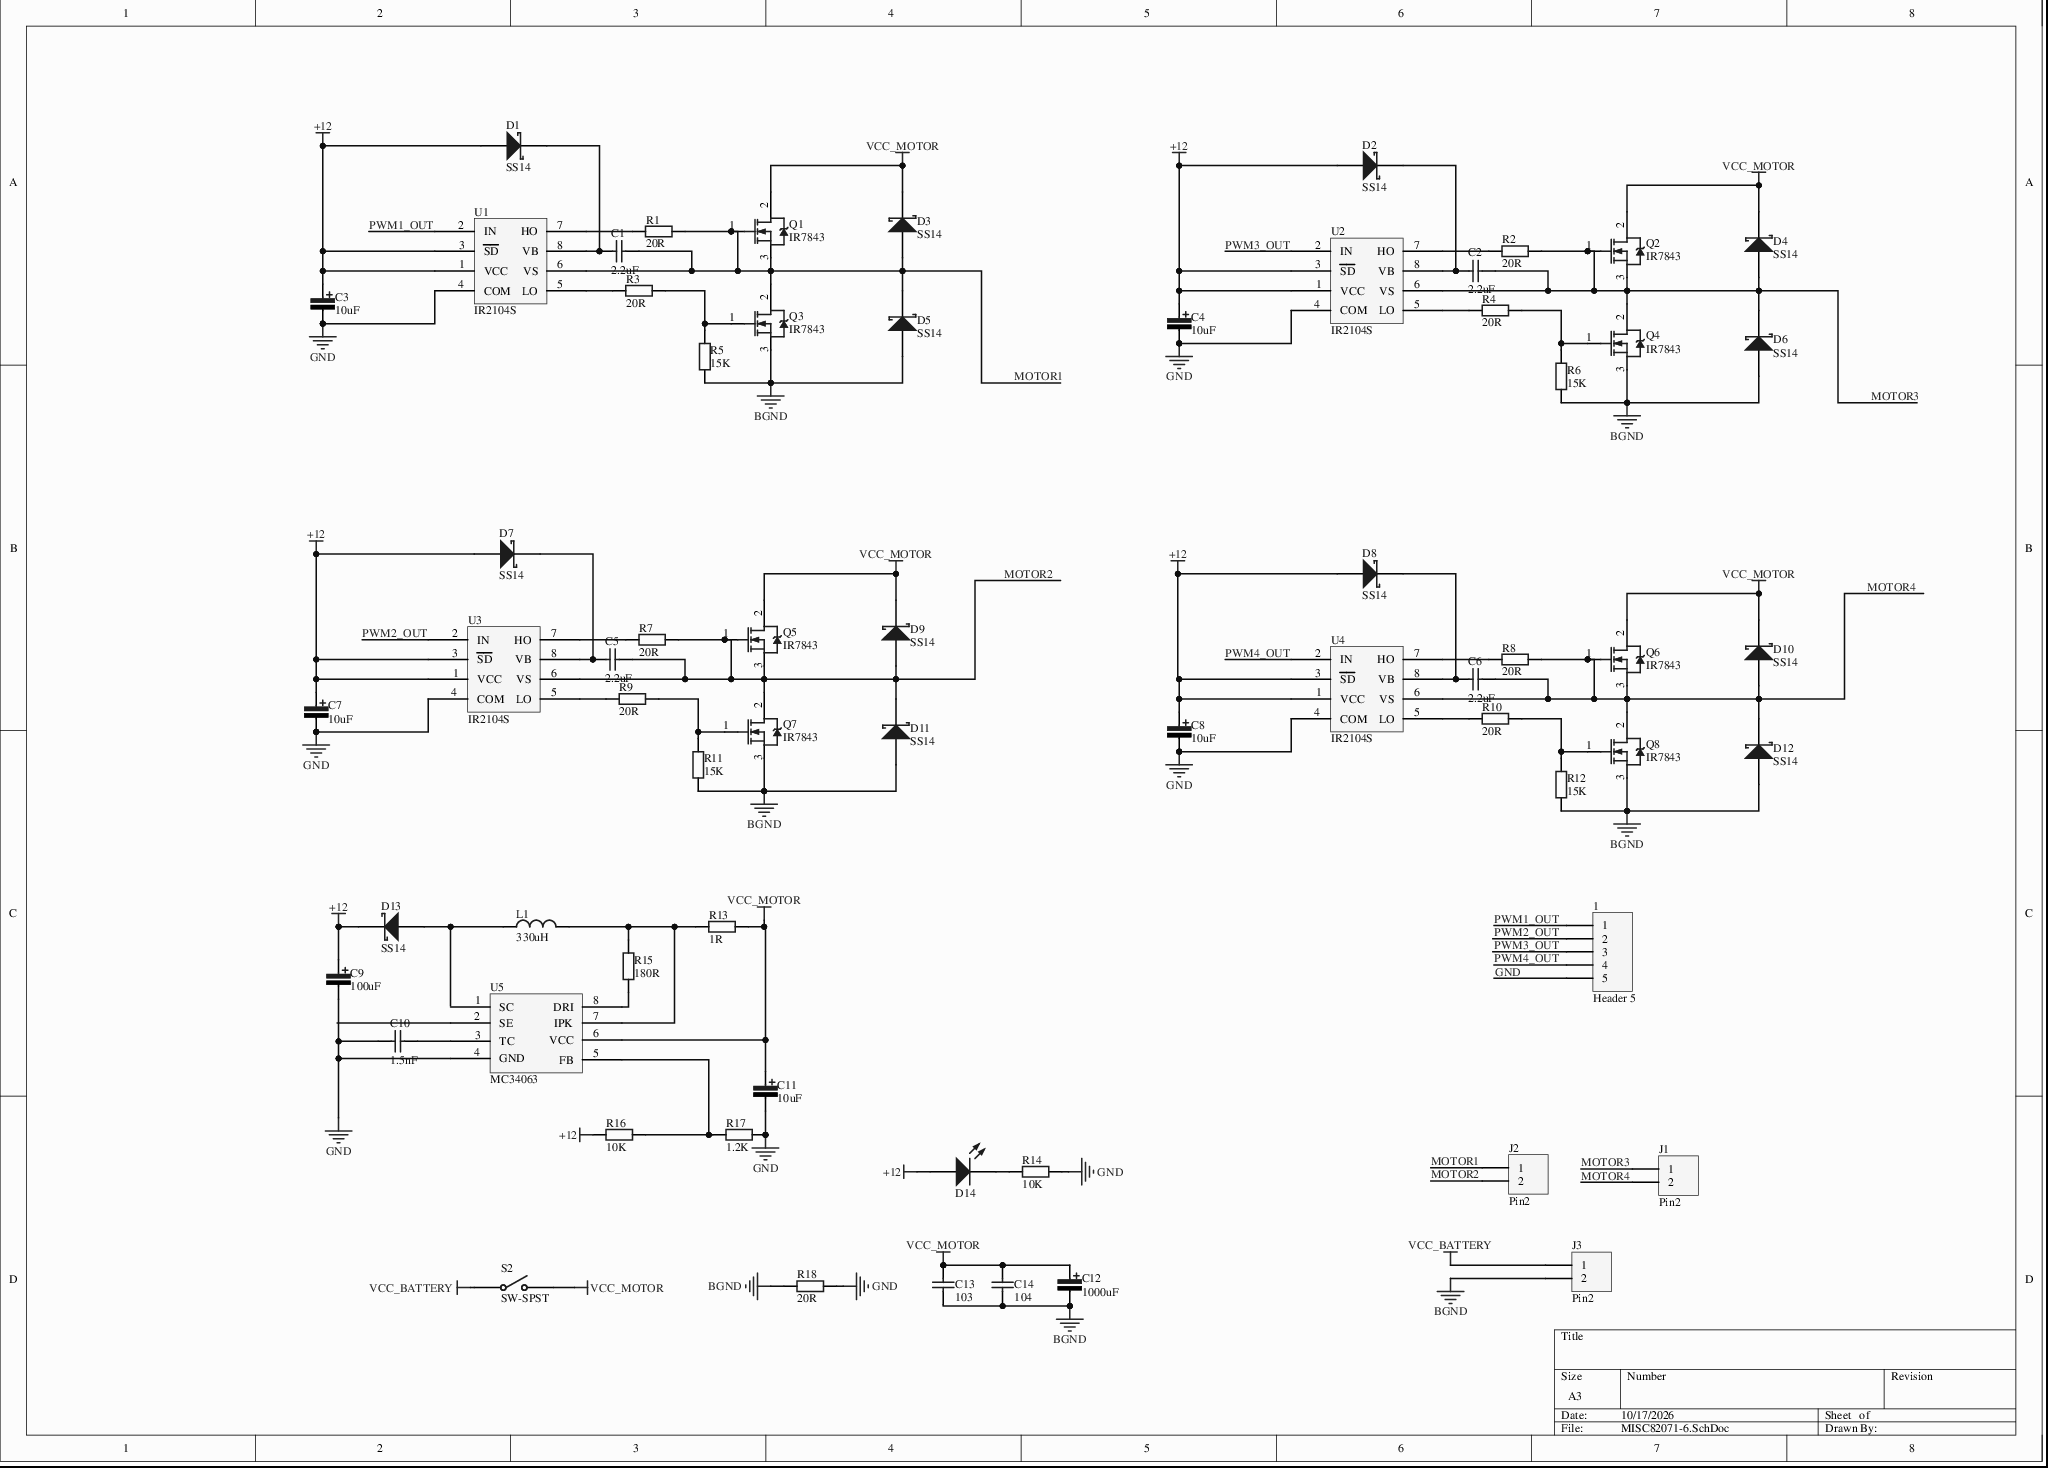
[diagram p0: MISC82071-6.SchDoc]
# Altium project MISC82071-6.PrjPcb
1 sheet, 65 parts. Net scope: global (net labels, ports and power ports of the same name join across sheets).
Board file: MISC82071.PcbDoc

## Sheet MISC82071-6.SchDoc
size A3; SheetNumber: 1; SheetTotal: 1

### Parts
1  Header 5  [HDR1X5]
C1  value 2.2uF  [my0603]  (hidden comment: Cap)
C2  value 2.2uF  [my0603]  (hidden comment: Cap)
C3  value 10uF  [CAP-3528]  (hidden comment: Cap Pol)
C4  value 10uF  [CAP-3528]  (hidden comment: Cap Pol)
C5  value 2.2uF  [my0603]  (hidden comment: Cap)
C6  value 2.2uF  [my0603]  (hidden comment: Cap)
C7  value 10uF  [CAP-3528]  (hidden comment: Cap Pol)
C8  value 10uF  [CAP-3528]  (hidden comment: Cap Pol)
C9  value 100uF  [CAP-3528]  (hidden comment: Cap Pol)
C10  value 1.5nF  [my0603]  (hidden comment: Cap)
C11  value 10uF  [CAP-3528]  (hidden comment: Cap Pol)
C12  value 1000uF  [CM A(3*5.4)]  (hidden comment: Cap Pol)
C13  value 103  [my0603]  (hidden comment: Cap)
C14  value 104  [my0603]  (hidden comment: Cap)
D1  Type: SS14  [DIODE-SMA]  (hidden comment: D-Schottky)
D2  Type: SS14  [DIODE-SMA]  (hidden comment: D-Schottky)
D3  Type: SS14  [DIODE-SMA]  (hidden comment: D-Schottky)
D4  Type: SS14  [DIODE-SMA]  (hidden comment: D-Schottky)
D5  Type: SS14  [DIODE-SMA]  (hidden comment: D-Schottky)
D6  Type: SS14  [DIODE-SMA]  (hidden comment: D-Schottky)
D7  Type: SS14  [DIODE-SMA]  (hidden comment: D-Schottky)
D8  Type: SS14  [DIODE-SMA]  (hidden comment: D-Schottky)
D9  Type: SS14  [DIODE-SMA]  (hidden comment: D-Schottky)
D10  Type: SS14  [DIODE-SMA]  (hidden comment: D-Schottky)
D11  Type: SS14  [DIODE-SMA]  (hidden comment: D-Schottky)
D12  Type: SS14  [DIODE-SMA]  (hidden comment: D-Schottky)
D13  Type: SS14  [DIODE-SMA]  (hidden comment: D-Schottky)
D14  LED0  [0805]  (value not drawn)
J1  Pin2  [PCBComponent_1 - duplicate]
J2  Pin2  [PCBComponent_1 - duplicate]
J3  Pin2  [PCBComponent_1 - duplicate]
L1  value 330uH  [L-SMD-7]  (hidden comment: Inductor)
Q1  IR7843  [LR7843]
Q2  IR7843  [LR7843]
Q3  IR7843  [LR7843]
Q4  IR7843  [LR7843]
Q5  IR7843  [LR7843]
Q6  IR7843  [LR7843]
Q7  IR7843  [LR7843]
Q8  IR7843  [LR7843]
R1  value 20R  [0805]  (hidden comment: Res1)
R2  value 20R  [0805]  (hidden comment: Res1)
R3  value 20R  [0805]  (hidden comment: Res1)
R4  value 20R  [0805]  (hidden comment: Res1)
R5  value 15K  [0805]  (hidden comment: Res1)
R6  value 15K  [0805]  (hidden comment: Res1)
R7  value 20R  [0805]  (hidden comment: Res1)
R8  value 20R  [0805]  (hidden comment: Res1)
R9  value 20R  [0805]  (hidden comment: Res1)
R10  value 20R  [0805]  (hidden comment: Res1)
R11  value 15K  [0805]  (hidden comment: Res1)
R12  value 15K  [0805]  (hidden comment: Res1)
R13  value 1R  [0805]  (hidden comment: Res1)
R14  value 10K  [0805]  (hidden comment: Res1)
R15  value 180R  [0805]  (hidden comment: Res1)
R16  value 10K  [0805]  (hidden comment: Res1)
R17  value 1.2K  [0805]  (hidden comment: Res1)
R18  value 20R  [0805]  (hidden comment: Res1)
S2  SW-SPST  [SWITCH]
U1  IR2104S  [IR2104]
U2  IR2104S  [IR2104]
U3  IR2104S  [IR2104]
U4  IR2104S  [IR2104]
U5  MC34063  [MC34063]

### Nets
+12: C3.1 C4.1 C7.1 C8.1 C9.1 D1.1(A) D2.1(A) D7.1(A) D8.1(A) D13.2(K) D14.1(A) R16.1 U1.1(VCC) U1.3(~{SD}) U2.1(VCC) U2.3(~{SD}) U3.1(VCC) U3.3(~{SD}) U4.1(VCC) U4.3(~{SD})
BGND: C12.2 C13.1 C14.1 D5.1(A) D6.1(A) D11.1(A) D12.1(A) J3.2 Q3.3(S) Q4.3(S) Q7.3(S) Q8.3(S) R5.1 R6.1 R11.1 R12.1 R18.1
GND: 1.5 C3.2 C4.2 C7.2 C8.2 C9.2 C10.1 C11.2 R14.2 R17.2 R18.2 U1.4(COM) U2.4(COM) U3.4(COM) U4.4(COM) U5.4(GND)
VCC_BATTERY: J3.1 S2.1(COMMON)
VCC_MOTOR: C11.1 C12.1 C13.2 C14.2 D3.2(K) D4.2(K) D9.2(K) D10.2(K) Q1.2(D) Q2.2(D) Q5.2(D) Q6.2(D) R13.2 S2.2(NO) U5.6(VCC)
MOTOR1: C1.2 D3.1(A) D5.2(K) J2.1 Q1.1(G) Q1.3(S) Q3.2(D) R1.2 U1.6(VS)
MOTOR2: C5.2 D9.1(A) D11.2(K) J2.2 Q5.1(G) Q5.3(S) Q7.2(D) R7.2 U3.6(VS)
MOTOR3: C2.2 D4.1(A) D6.2(K) J1.1 Q2.1(G) Q2.3(S) Q4.2(D) R2.2 U2.6(VS)
MOTOR4: C6.2 D10.1(A) D12.2(K) J1.2 Q6.1(G) Q6.3(S) Q8.2(D) R8.2 U4.6(VS)
PWM1_OUT: 1.1 U1.2(IN)
PWM2_OUT: 1.2 U3.2(IN)
PWM3_OUT: 1.3 U2.2(IN)
PWM4_OUT: 1.4 U4.2(IN)
NetC1_1: C1.1 D1.2(K) U1.8(VB)
NetC2_1: C2.1 D2.2(K) U2.8(VB)
NetC5_1: C5.1 D7.2(K) U3.8(VB)
NetC6_1: C6.1 D8.2(K) U4.8(VB)
NetC10_2: C10.2 U5.3(TC)
NetD13_1: D13.1(A) L1.1
NetD14_2: D14.2(K) R14.1
NetL1_2: L1.2 R13.1 R15.2 U5.7(IPK)
NetQ3_1: Q3.1(G) R3.2 R5.2
NetQ4_1: Q4.1(G) R4.2 R6.2
NetQ7_1: Q7.1(G) R9.2 R11.2
NetQ8_1: Q8.1(G) R10.2 R12.2
NetR1_1: R1.1 U1.7(HO)
NetR2_1: R2.1 U2.7(HO)
NetR3_1: R3.1 U1.5(LO)
NetR4_1: R4.1 U2.5(LO)
NetR7_1: R7.1 U3.7(HO)
NetR8_1: R8.1 U4.7(HO)
NetR9_1: R9.1 U3.5(LO)
NetR10_1: R10.1 U4.5(LO)
NetR15_1: R15.1 U5.8(DRI)
NetR16_2: R16.2 R17.1 U5.5(FB)

Not connected (* = marked no-connect by the designer): U5 1(SC) 2(SE)

### Library data of the parts
1 = Header 5: Header, 5-Pin; LatestRevisionDate: 17-Jul-2002; LatestRevisionNote: Re-released for DXP Platform.; Publisher: Altium Limited
C1 C2 C5 C6 C10 C13 C14 = Cap: Non-polarized capacitor; Published: 8-Jun-2000; LatestRevisionDate: 17-Jul-2002; LatestRevisionNote: Re-released for DXP Platform.; PackageReference: RAD-0.3; Publisher: Altium Limited
C3 C4 C7-C9 C11 C12 = Cap Pol: Polarized electrolytic capacitor; Vol: 16V; Published: 8-Jun-2000; LatestRevisionDate: 17-Jul-2002; LatestRevisionNote: Re-released for DXP Platform.; PackageReference: RB7.6-15; Publisher: Altium Limited
D1-D13 = D-Schottky: Schottky diode; Published: 8-Jun-2000; LatestRevisionDate: 17-Jul-2002; LatestRevisionNote: Re-released for DXP Platform.; PackageReference: SMB; Code_JEDEC: DO-214-AA; Publisher: Altium Limited
D14 = LED0: LED; Published: 8-Jun-2000; LatestRevisionDate: 08-Jul-2005; LatestRevisionNote: Mech Layer 1 removed.; PackageReference: LED-0; Publisher: Altium Limited
L1 = Inductor: Code_IEC: 1005; Published: 8-Jun-2000; LatestRevisionDate: 17-Jul-2002; LatestRevisionNote: Re-released for DXP Platform.; Code_JEITA: 0402; Publisher: Altium Limited
Q1-Q8 = NMOS: N-Channel Power MOSFET; Note: Pin 2 is electrically connected to pin 4.; Published: 8-Jun-2000; LatestRevisionDate: 17-Jul-2002; LatestRevisionNote: Re-released for DXP Platform.; DatasheetVersion: PD-9.814; PackageVersion: Feb-1997; PackageReference: TO-220AB; PackageDescription: TO, Thru-Hole, Vertical, Heatsink Mounted; 3 In-Line Leads; Pitch 2.54 mm; ComponentLink1Description: Manufacturer Link; Publisher: Altium Limited
R1-R18 = Res1: Chip resistor; Published: 8-Jun-2000; LatestRevisionDate: 17-Jul-2002; LatestRevisionNote: Re-released for DXP Platform.; PackageReference: AXIAL-0.4; Publisher: Altium Limited
S2 = SW-SPST: Single-Pole, Single-Throw Switch; Published: 24-Mar-1999; LatestRevisionDate: 17-Jul-2002; LatestRevisionNote: Re-released for DXP Platform.; PackageReference: SPST-2; PackageDescription: Switch; 2 Leads; Publisher: Altium Limited
U1-U4 = IR2104